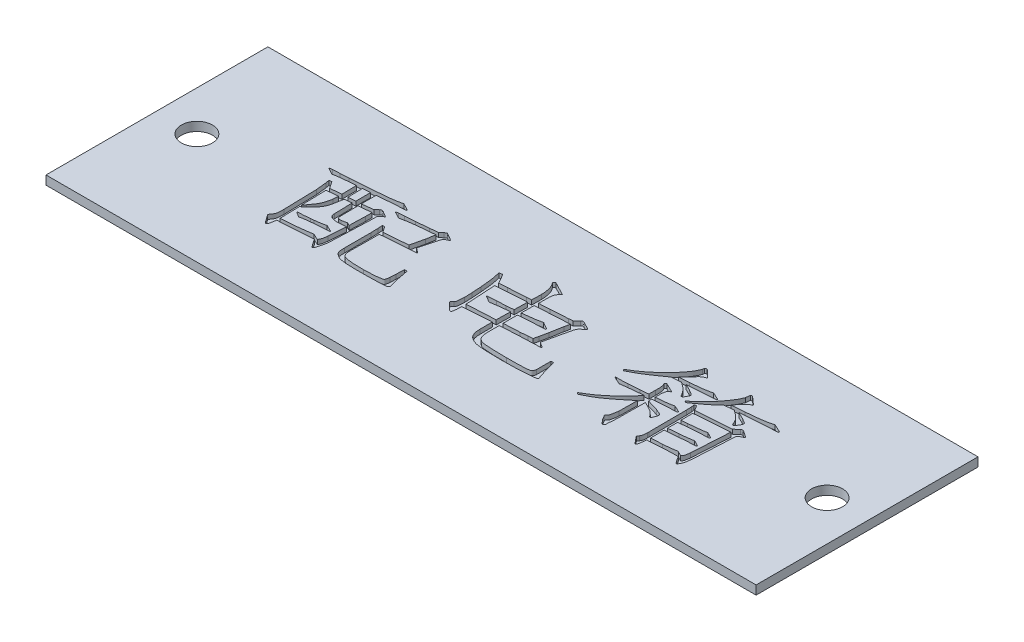
SolidWorks part; units mm, degrees
ref_plane "前视基准面" through (0, 0, 0) normal (0, 0, 1) x (1, 0, 0)
ref_plane "上视基准面" through (0, 0, 0) normal (0, 1, 0) x (1, 0, 0)
ref_plane "右视基准面" through (0, 0, 0) normal (1, 0, 0) x (0, 0, -1)
sketch "草图1" plane through (0, 0, 0) normal (0, 1, 0) x (1, 0, 0)
  line L1 (-40, -12.5) -> (40, -12.5)
  line L2 (-40, -12.5) -> (-40, 12.5)
  line L3 (-40, 12.5) -> (40, 12.5)
  line L4 (40, -12.5) -> (40, 12.5)
  line L5 (-40, -12.5) -> (40, 12.5) construction
  line L6 (-40, 12.5) -> (40, -12.5) construction
  circle A0 centre (-35.5, 0) radius 1.75
  circle A1 centre (35.5, 0) radius 1.75
  point P0 (0, 0)
  dimension "D3" = 3.5
  dimension "D4" = 3.5
  dimension "D5" = 71
  dimension "D6" = 35.5
  dimension "D1" = 80
  dimension "D2" = 25
extrude "凸台-拉伸1" add sketch "草图1" along normal blind 1
sketch "草图2" plane through (0, 1, 0) normal (0, 1, 0) x (1, 0, 0)
  text T0 "配电箱" font "汉仪长仿宋体" height 8
extrude "切除-拉伸1" cut sketch "草图2" against normal blind 0.5
